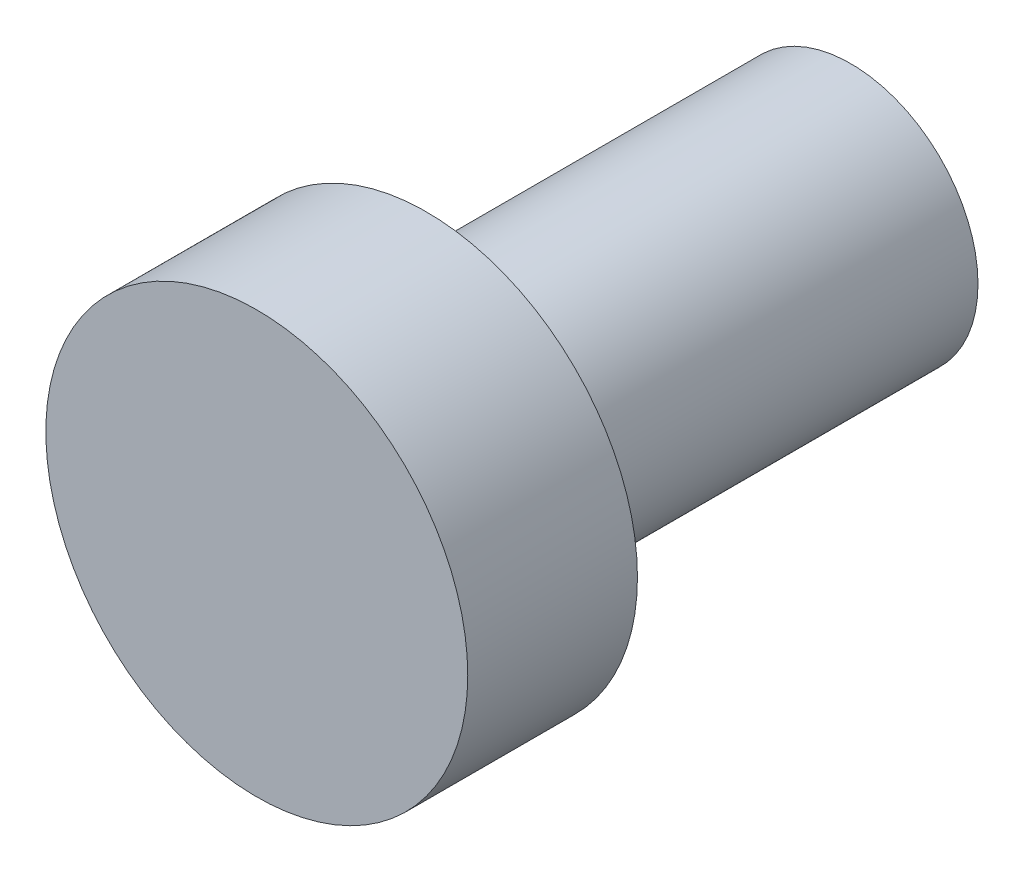
from build123d import *

# Parameters (mm, degrees)
SKETCH1_R           = 1.5
BOSS_EXTRUDE1_DEPTH = 5
SKETCH2_R           = 2.486398422
BOSS_EXTRUDE2_DEPTH = 2


with BuildPart() as part:
    # Sketch1 → Boss-Extrude1 (new body)
    with BuildSketch(Plane.XY):
        with Locations((-45.197762361, 32.025823543)):
            Circle(SKETCH1_R)
    extrude(amount=-BOSS_EXTRUDE1_DEPTH)

    # Sketch2 → Boss-Extrude2 (add)
    with BuildSketch(Plane.XY):
        with Locations((-45.197762361, 32.025823543)):
            Circle(SKETCH2_R)
    extrude(amount=BOSS_EXTRUDE2_DEPTH)


solid = part.part
